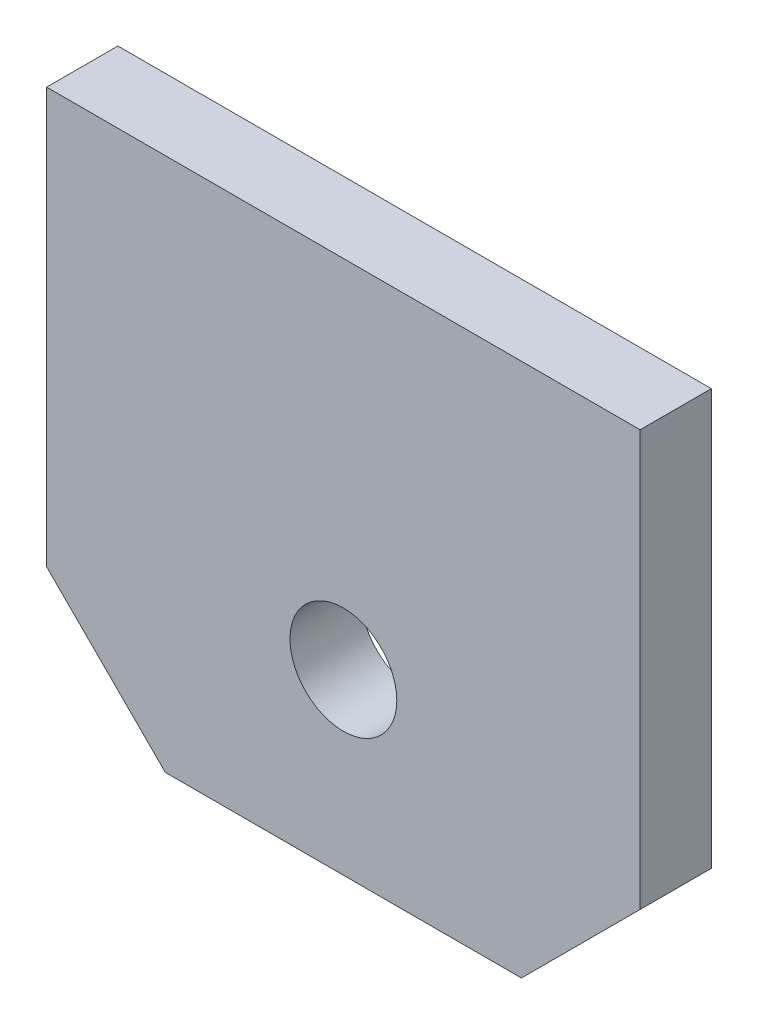
from build123d import *

# Parameters (mm, degrees)
SKETCH1_W           = 50
SKETCH1_H           = 45
BOSS_EXTRUDE1_DEPTH = 6
SKETCH2_R           = 4.5
CUT_EXTRUDE1_DEPTH  = 6
CHAMFER1_SIZE       = 10


with BuildPart() as part:
    # Sketch1 → Boss-Extrude1 (new body)
    with BuildSketch(Plane.XY):
        Rectangle(SKETCH1_W, SKETCH1_H)
    extrude(amount=BOSS_EXTRUDE1_DEPTH)

    # Sketch2 → Cut-Extrude1 (cut)
    with BuildSketch(Plane.XY.offset(6)):
        with Locations((0, -7.5)):
            Circle(SKETCH2_R)
    extrude(amount=-CUT_EXTRUDE1_DEPTH, mode=Mode.SUBTRACT)

    # Chamfer1
    chamfer1_edges = [part.edges().sort_by_distance(p)[0] for p in [
        (25, -22.5, 3),
        (-25, -22.5, 3),
    ]]
    chamfer(chamfer1_edges, length=CHAMFER1_SIZE)


solid = part.part
